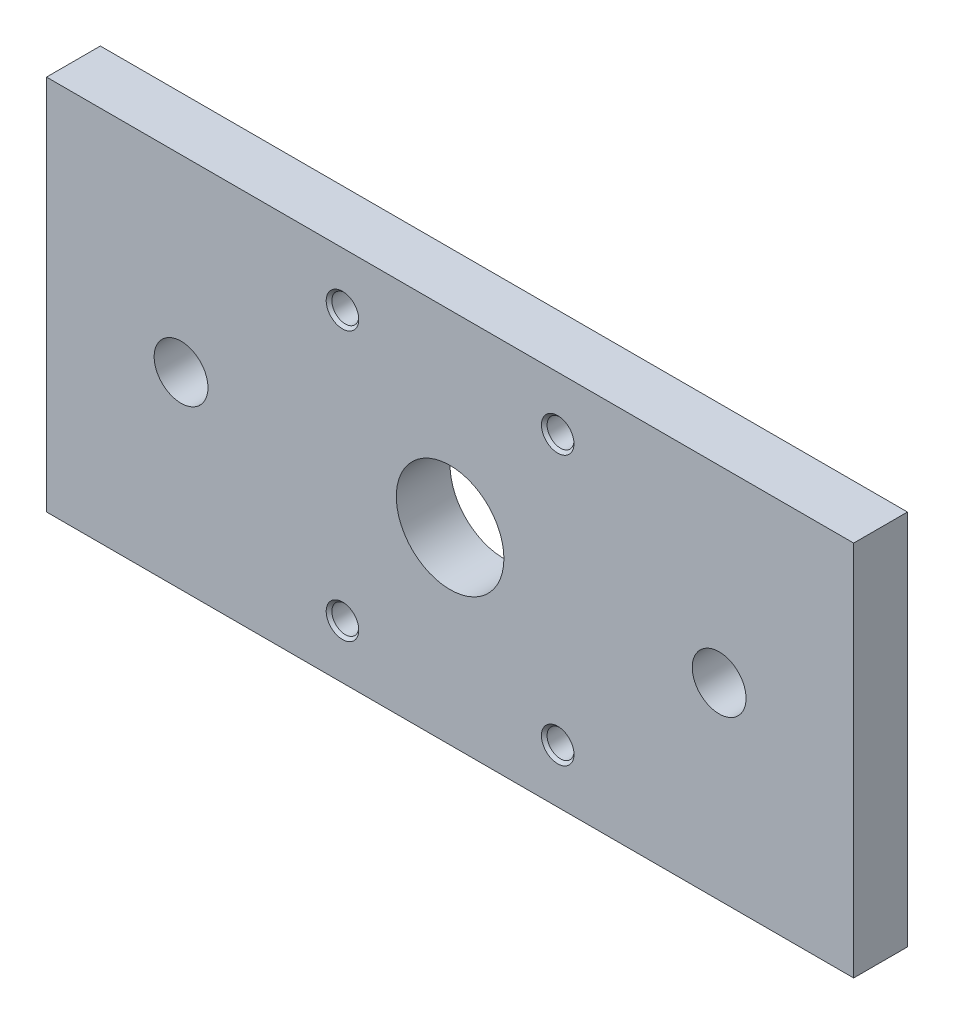
from build123d import *

# Parameters (mm, degrees)
SKETCH_1_W                   = 150
SKETCH_1_H                   = 70
EXTRUDE_1_DEPTH              = 10
SKETCH_2_R                   = 10
CUT_EXTRUDE_1_DEPTH          = 55
SKETCH_7_R                   = 5
CUT_EXTRUDE_2_DEPTH          = 20
HOLE_WIZARD_M6_1_D           = 5
HOLE_WIZARD_M6_1_DEPTH       = 13.497848452
HOLE_WIZARD_M6_1_CSINK_D     = 6.05
HOLE_WIZARD_M6_1_CSINK_ANGLE = 90
HOLE_WIZARD_M6_1_TIP         = 1.502151548


with BuildPart() as part:
    # 草图1 → 凸台-拉伸1 (new body)
    with BuildSketch(Plane.XY):
        Rectangle(SKETCH_1_W, SKETCH_1_H)
    extrude(amount=EXTRUDE_1_DEPTH)

    # 草图2 → 切除-拉伸1 (cut)
    with BuildSketch(Plane.XY.offset(10)):
        Circle(SKETCH_2_R)
    extrude(amount=-CUT_EXTRUDE_1_DEPTH, mode=Mode.SUBTRACT)

    # 草图7 → 切除-拉伸2 (cut)
    with BuildSketch(Plane.XY.offset(10)):
        with Locations((-50, 0)):
            Circle(SKETCH_7_R)
        with Locations((50, 0)):
            Circle(SKETCH_7_R)
    extrude(amount=-CUT_EXTRUDE_2_DEPTH, mode=Mode.SUBTRACT)

    # M6 螺纹孔1
    with Locations(Plane.XY.offset(10)):
        with Locations((20, 25), (-20, 25), (-20, -25), (20, -25)):
            CounterSinkHole(HOLE_WIZARD_M6_1_D / 2, HOLE_WIZARD_M6_1_CSINK_D / 2, depth=HOLE_WIZARD_M6_1_DEPTH, counter_sink_angle=HOLE_WIZARD_M6_1_CSINK_ANGLE)
            with Locations((0, 0, -(HOLE_WIZARD_M6_1_DEPTH + HOLE_WIZARD_M6_1_TIP / 2))):  # 118° drill point
                Cone(0, HOLE_WIZARD_M6_1_D / 2, HOLE_WIZARD_M6_1_TIP, mode=Mode.SUBTRACT)


solid = part.part
